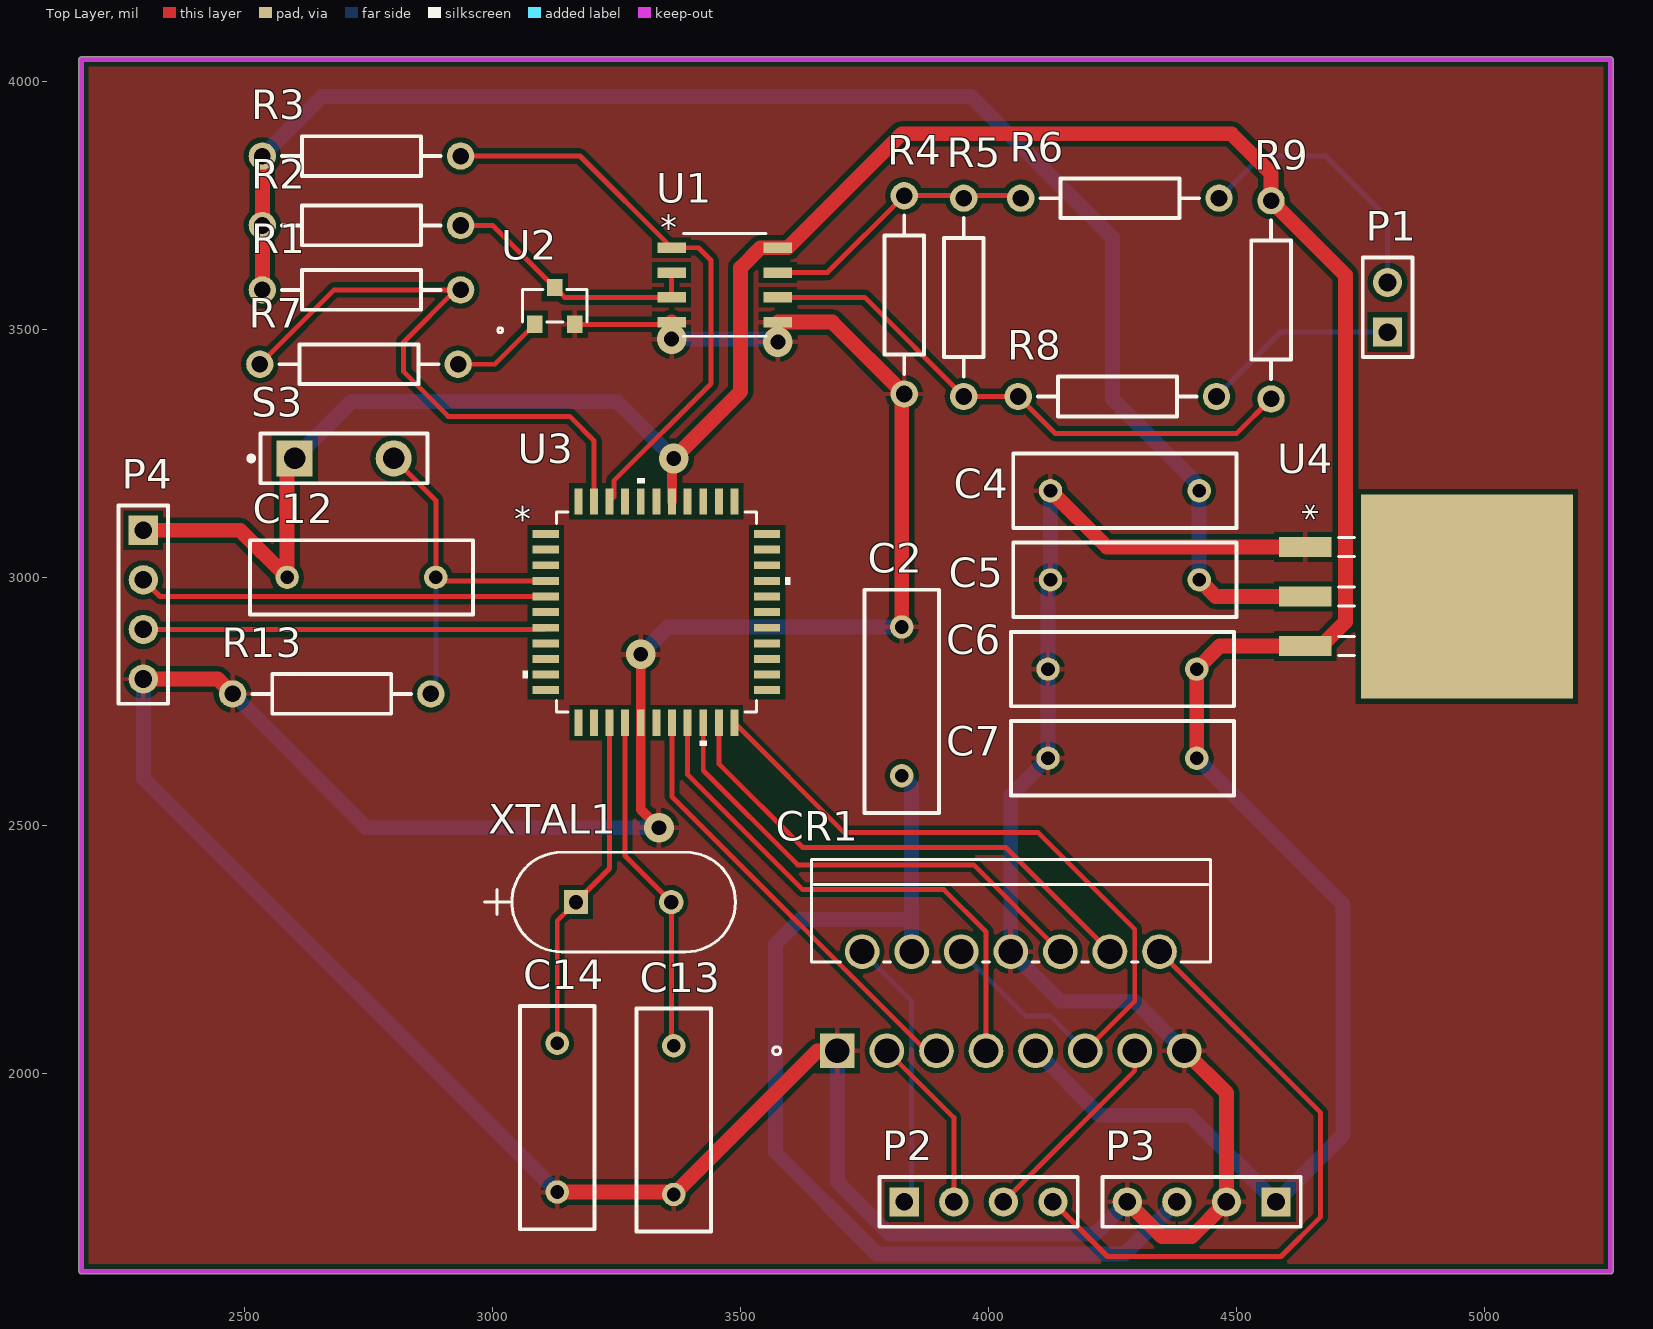
[diagram p0: Top Layer view]
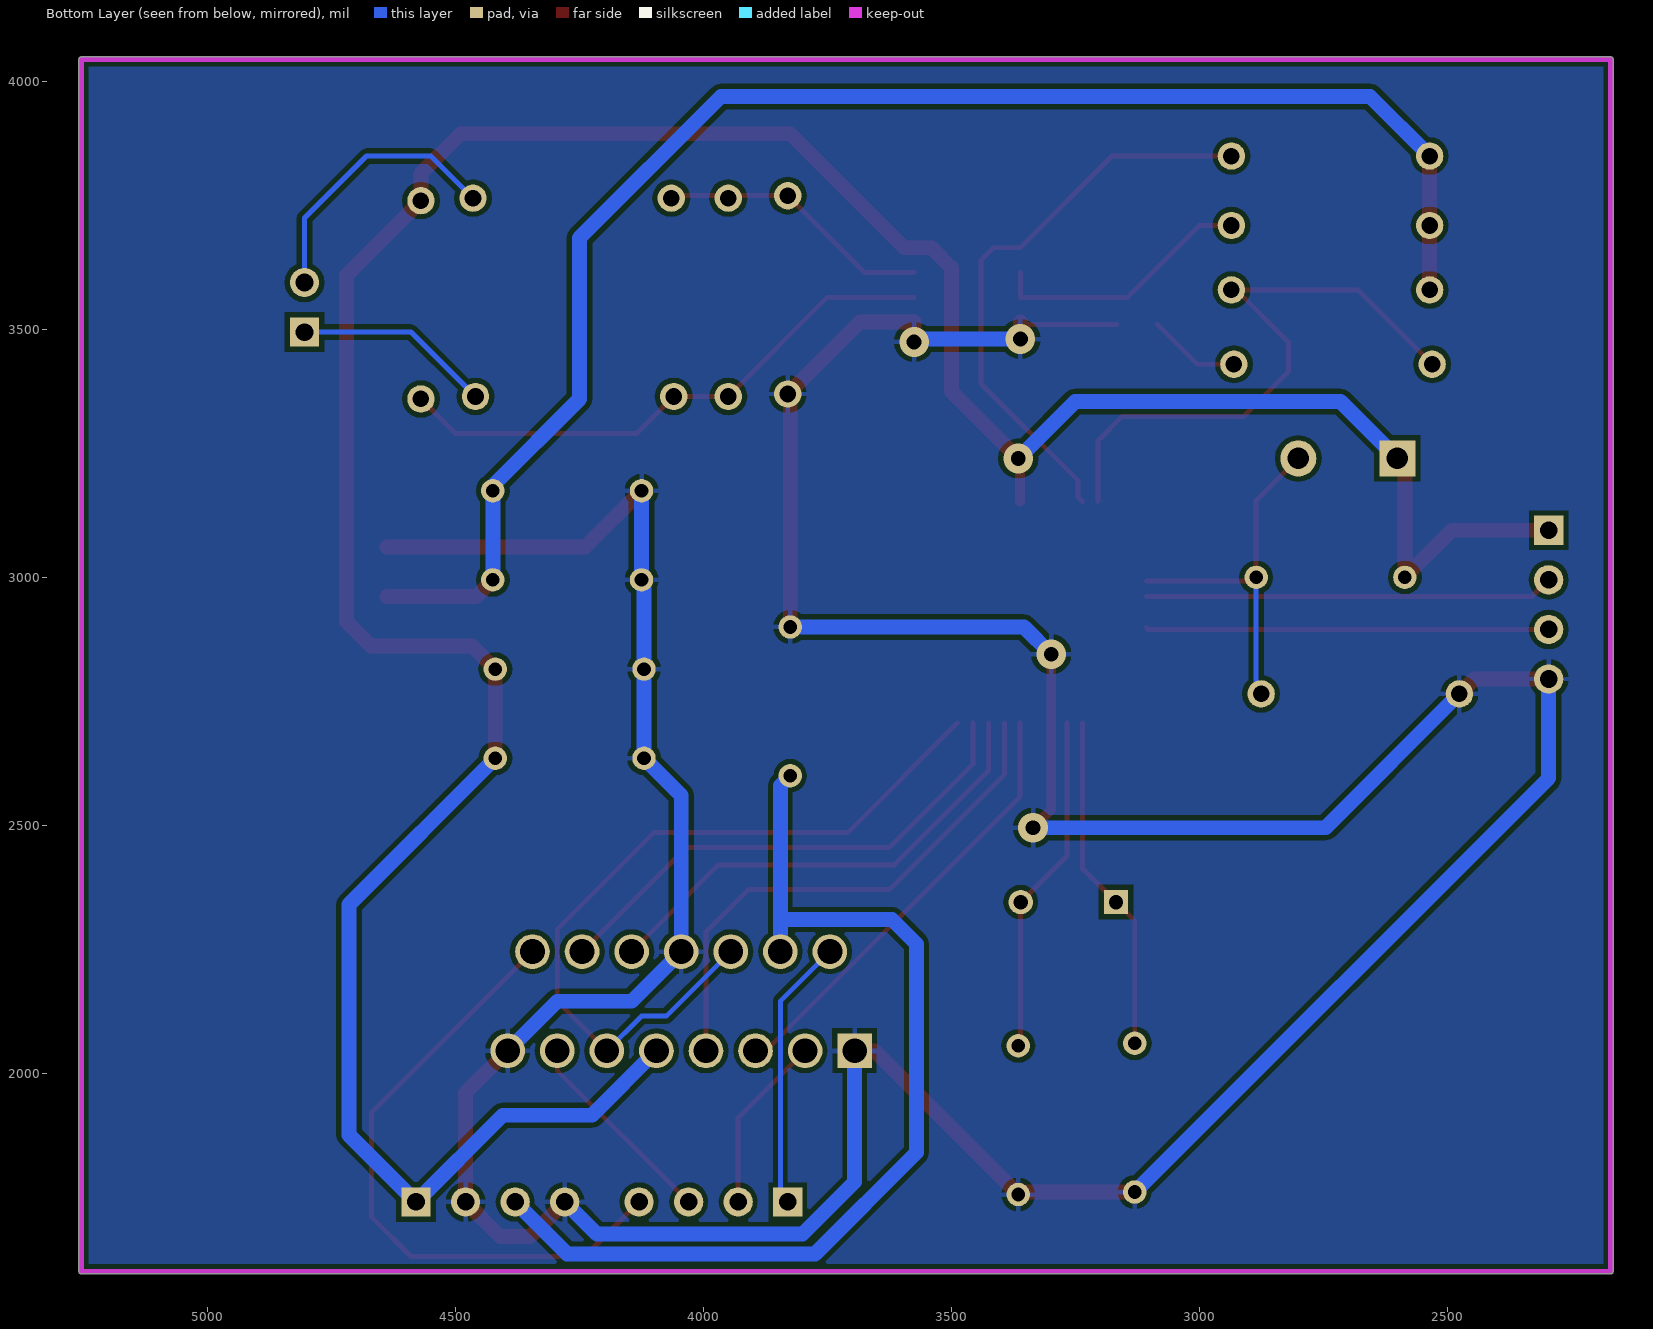
[diagram p1: Bottom Layer view, seen from below]
# Altium PCB MISC76236.PcbDoc
Units mil, origin at the board's own origin, x right, y up, seen from the top; angles counter-clockwise.
Board outline 3095.03 x 2455.03 mil, 2 copper layers (Top Layer, Bottom Layer); 29 components, 26 nets, 128 pads, 5 vias.

## Layer stack, top to bottom (the 12.6 mil dielectric is the usual default, probably not edited)
Top Solder: solder mask 0.4, Solder Resist, Dk 3.5
Top Layer: signal copper 1.4
Dielectric 1: dielectric 12.6, FR-4, Dk 4.8
Bottom Layer: signal copper 1.4
Bottom Solder: solder mask 0.4, Solder Resist, Dk 3.5

## Board outline
2164.99,1600 ccw(c2170,1600) 2170,1594.98 5255,1594.98 ccw(c5255,1600) 5260.02,1600 5260.02,4045 ccw(c5255,4045) 5255,4050.01 2170,4050.01 ccw(c2170,4045) 2164.99,4045

## Design rules (kind name [scope] priority, off if disabled: settings)
Clearance [All] p1: gap=10
MinimumSolderMaskSliver [All] p1: minsoldermaskwidth=0
PolygonConnect [All] p1: connectstyle=Relief reliefconductorwidth=10 reliefentries=4 polygonreliefangle="90 Angle" airgapwidth=10
RoutingVias [All] p1: holewidth=28 width=50 viastyle="Through Hole" minholewidth=28 minwidth=50 maxholewidth=28 maxwidth=50
SilkToSilkClearance [All] p1: silktosilkclearance=0
SilkToSolderMaskClearance [IsPad] p1: minsilkscreentomaskgap=0 clearancetoexposedcopper=TRUE
SolderMaskExpansion [All] p1: expansion=4
Width [All] p1: maxlimit=30 minlimit=10 preferedwidth=10
27 further rules are at their usual default settings.

## Components (designator, comment, footprint, x,y, rotation, side; value= is the part's Value field where it differs from the comment)
C2 "Cap" RAD-0.3 3825,2750 r270 top
C4 "Cap" RAD-0.3 4275,3175 r0 top
C5 "Cap" RAD-0.3 4275,2995 r0 top
C6 "Cap" RAD-0.3 4270,2815 r0 top
C7 "Cap" RAD-0.3 4270,2635 r0 top
C12 "Cap" RAD-0.3 2735,3000 r0 top
C13 "Cap" RAD-0.3 3365,1905 r90 top
C14 "Cap" RAD-0.3 3130,1910 r90 top
CR1 "L298N" Multiwatt15_V_STM 3695,2045 r0 top
P1 "Header 2" HDR1X2 4805,3495 r90 top
P2 "Header 4" HDR1X4 3830,1740 r0 top
P3 "Header 4" HDR1X4 4580,1740 r180 top
P4 "Header 4" HDR1X4 2295,3095 r270 top
R1 "Res2" AXIAL-0.4 2735,3580 r180 top
R2 "Res2" AXIAL-0.4 2735,3710 r180 top
R3 "Res2" AXIAL-0.4 2735,3850 r180 top
R4 "Res2" AXIAL-0.4 3830,3570 r270 top
R5 "Res2" AXIAL-0.4 3950,3565 r90 top
R6 "Res2" AXIAL-0.4 4265,3765 r0 top
R7 "Res2" AXIAL-0.4 2730,3430 r0 top
R8 "Res2" AXIAL-0.4 4260,3365 r0 top
R9 "Res2" AXIAL-0.4 4570,3560 r270 top
R13 "Res2" AXIAL-0.4 2675,2765 r0 top
S3 "SW-PB" SPST-2 2700,3240 r0 top
U1 "MAX485CSA+" 21-0041B_8_MXM 3467.86,3590 r0 top
U2 "MMBT3904-7-F" SOT-23_1_DIO 3125,3547.8 r0 top
U3 "STC12C5A60S2-35I-LQFP44" LQFP44_STC89_STC_SCM 3330,2930 r0 top
U4 "AMS1117-3.3" TS3B_TEX 4965,2961.5 r270 top
XTAL1 "HC49S-11.0592-30-50-70-30-ATF" XTAL_HC49S_MTC 3167.87,2345 r0 top

## Footprints (in the part's own frame and the unit in brackets; to place one, negate y for a bottom-side part, rotate by r counter-clockwise, add the part's x,y. Pads: shape width x height; smd on the part's side, far side on the other; paste and mask are expansions set on the pad)
21-0041B_8_MXM [mil]
  rect 57.28x20.97 smd paste+0 mask+0: 1(-107.14,75) 2(-107.14,25) 3(-107.14,-25) 4(-107.14,-75) 5(107.14,-75) 6(107.14,-25) 7(107.14,25) 8(107.14,75)
  silkscreen extent -84,-104 84,104, body extent -122,-99 122,99, height 69
AXIAL-0.4 [mm] "Axial Device, Thru-Hole; 2 Leads; 0.4 in Pin Spacing"
  round 1.4 hole 0.85: 1(-5.08,0) 2(5.08,0)
  silkscreen extent -4.06,-1.02 4.06,1.02
HDR1X2 [mm] "Connector; Header; 2 Position"
  rect 1.5x1.5 hole 0.9: 1(0,0)
  round 1.5 hole 0.9: 2(2.54,0)
  silkscreen extent -1.27,-1.27 3.81,1.27
HDR1X4 [mm] "Connector; Header; 4 Position"
  rect 1.5x1.5 hole 0.9: 1(0,0)
  round 1.5 hole 0.9: 2(2.54,0) 3(5.08,0) 4(7.62,0)
  silkscreen extent -1.27,-1.27 8.89,1.27
LQFP44_STC89_STC_SCM [mil]
  rect 52.78x15.97 smd paste+0 mask+0: 1(-223.39,157.5) 2(-223.39,126) 3(-223.39,94.5) 4(-223.39,63) 5(-223.39,31.5) 6(-223.39,0) 7(-223.39,-31.5) 8(-223.39,-63) 9(-223.39,-94.5) 10(-223.39,-126) 11(-223.39,-157.5) 23(223.39,-157.5) 24(223.39,-126) 25(223.39,-94.5) 26(223.39,-63) 27(223.39,-31.5) 28(223.39,0) 29(223.39,31.5) 30(223.39,63) 31(223.39,94.5) 32(223.39,126) 33(223.39,157.5)
  rect 15.97x52.78 smd paste+0 mask+0: 12(-157.5,-223.39) 13(-126,-223.39) 14(-94.5,-223.39) 15(-63,-223.39) 16(-31.5,-223.39) 17(0,-223.39) 18(31.5,-223.39) 19(63,-223.39) 20(94.5,-223.39) 21(126,-223.39) 22(157.5,-223.39) 34(157.5,223.39) 35(126,223.39) 36(94.5,223.39) 37(63,223.39) 38(31.5,223.39) 39(0,223.39) 40(-31.5,223.39) 41(-63,223.39) 42(-94.5,223.39) 43(-126,223.39) 44(-157.5,223.39)
  silkscreen extent -270,-270 270,270, body extent -236,-236 236,236, height 63
Multiwatt15_V_STM [mil]
  rect 70x70 / inner round 60 / far side rect 70x70 hole 50 paste-35 mask+0: 1(0,0)
  round 70 / inner round 60 / far side round 70 hole 50 paste-35 mask+0: 2(50,200) 3(100,0) 4(150,200) 5(200,0) 6(250,200) 7(300,0) 8(350,200) 9(400,0) 10(450,200) 11(500,0) 12(550,200) 13(600,0) 14(650,200) 15(700,0)
  silkscreen extent -130,-8 752,386, body extent -48,-15 748,381, height 827
RAD-0.3 [mm] "Radial Cap, Thru-Hole; 2 Leads; 0.3 in Pin Spacing"
  round 1.2 hole 0.7: 1(-3.81,0) 2(3.81,0)
  silkscreen extent -5.71,-1.91 5.71,1.91
SOT-23_1_DIO [mil]
  rect 32x35 smd paste+0 mask+0: 1(-40.35,-37.2) 2(40.35,-37.2) 3(0,37.2)
  silkscreen extent -115,-54 65,33
SPST-2 [mm] "Switch; 2 Leads"
  rect 1.85x1.85 hole 1.1: 1(-2.54,0)
  round 1.85 hole 1.1: 2(2.54,0)
  silkscreen extent -4.89,-1.27 4.28,1.27
TS3B_TEX [mil]
  rect 39.97x105.56 smd paste+0 mask+0: 1(-100,-326) 2(0,-326) 3(100,-326)
  rect 412x428 smd paste+0 mask+0: 4(0,0)
  silkscreen extent -119,-259 119,-227, body extent -205,-278 205,200, height 189
XTAL_HC49S_MTC [mil]
  rect 49x49 / inner round 60 / far side rect 49x49 hole 29 paste-24.5 mask+0: 1(0,0)
  round 49 / inner round 60 / far side round 49 hole 29 paste-24.5 mask+0: 2(192.13,0)
  silkscreen extent -184,-100 322,100, body extent -134,-105 326,105, height 157

## Part data
C2 C4 C5 C6 C7 C12 C13 C14: "Capacitor"
CR1 U1 U2 U3 U4 XTAL1: "No Description Available"
P1: "Header, 2-Pin"
P2 P3 P4: "Header, 4-Pin"
R1 R2 R3 R4 R5 R6 R7 R8 R9 R13: "Resistor"
S3: "Switch"

## Via types
v1: diameter 60, hole 30, Top Layer to Bottom Layer, 5 vias

## Nets (pads, with @x,y where several pads share a name; then routed paths per layer and width w, separated by ;. In a path a pad name is that pad's centre, name@x,y a point inside that pad or via, vN(x,y) a via of type N, cw(c..) or ccw(c..) an arc to the next point about the centre after c; other vN are vias at no path point)
"485 RX": R3.1 U1.1 U3.42 | length 1163.3
  Top Layer w10: R3.1 3175.72,3850 U1.1 3415,3665 3440,3640 3440,3390.76 3244.02,3194.78 3244.02,3161.91 U3.42
"485 TX": R1.1 R7.1 U3.43 | length 1239.8
  Top Layer w10: R7.1 2680,3580 R1.1@2925,3580 ; R1.1 R1.1@2925,3580 ; U3.43 3204,3276 3155,3325 2910,3325 2820,3415 2820,3475 R1.1@2925,3580
+3.3: C4.2 C5.2 R1.2 R2.2 R3.2 U4.2 | length 3143.1
  Top Layer w30: R1.2 R2.2 R3.2 ; C5.2 4458.5,2961.5 U4.2
  Bottom Layer w30: R3.2 2655,3970 3965,3970 4250,3685 4250,3360 4425,3185 C4.2 C5.2
+5: C6.2 C7.2 C12.1 CR1.9 P3.1 P4.1 R9.1 S3.1 U1.8 U3.38 U4.3 | length 6350.7
  Top Layer w20: U3.38 v1@3361.5,3236.5
  Top Layer w30: P4.1 2490,3095 C12.1 2585,3225 S3.1 ; v1@3361.5,3236.5 v1(3365,3240) 3500,3375 3500,3625 3540,3665 U1.8 3595,3665 3825,3895 4490,3895 4570,3815 R9.1 4720,3610 4720,2910 4671.5,2861.5 U4.3 4466.5,2861.5 C6.2 C7.2
  Bottom Layer w30: S3.1 2715,3355 3250,3355 v1(3365,3240) ; CR1.9 4225,1915 4405,1915 P3.1 4715,1875 4715,2340 C7.2
+12: C2.2 CR1.4 P3.3 | length 2017.4
  Bottom Layer w30: C2.2 3845,2580 3845,2310 ; CR1.4 3845,2310 ; P3.3 4275,1635 3775,1635 3570,1840 3570,2260 3620,2310 3845,2310
A: P1.1 R8.2 | length 398.8
  Bottom Layer w10: R8.2 4590,3495 P1.1
A+: CR1.2 P2.1 | length 552.6
  Bottom Layer w10: CR1.2 3845,2145 3845,1755 P2.1
A-: CR1.3 P2.2 | length 360.9
  Top Layer w10: CR1.3 3930,1910 P2.2
B: P1.2 R6.2 | length 557
  Bottom Layer w10: R6.2 4550,3850 4680,3850 4805,3725 P1.2
B+: CR1.13 P2.3 | length 414.8
  Top Layer w10: P2.3 4295,2005 CR1.13
B-: CR1.14 P2.4 | length 1288.3
  Top Layer w10: P2.4 4240,1630 4590,1630 4670,1710 4670,1920 CR1.14
GND: C2.1 C4.1 C5.1 C6.1 C7.1 C13.1 C14.1 CR1.1 CR1.8 CR1.15 P3.2 P3.4 P4.4 R4.2 R13.1 U1.4 U1.5 U2.2 U3.16 U4.1 | length 8897.2
  Top Layer w10: U2.2 3356.31,3510.59 U1.4
  Top Layer w20: v1(3298.5,2845) U3.16 3298.5,2531.5 v1(3335,2495)
  Top Layer w30: P4.4 2445,2795 R13.1 ; C14.1 3360,1760 C13.1 3655,2045 CR1.1 ; v1(3360.72,3480.78) U1.4 ; v1(3575,3475) U1.5 3685,3515 R4.2 3825,3365 C2.1 ; C4.1 4238.5,3061.5 U4.1 ; P3.4 4350,1670 4410,1670 P3.2 4480,1960 CR1.15
  Bottom Layer w30: P4.4 2295,2595 C14.1 ; R13.1 2745,2495 v1(3335,2495) ; v1(3298.5,2845) 3353.5,2900 C2.1 ; v1(3360.72,3480.78) 3569.22,3480.78 v1(3575,3475) ; CR1.1 3695,1780.59 3800.59,1675 4215,1675 P3.4 ; C4.1 C5.1 4120,2990 C6.1 C7.1 4045,2560 CR1.8 4145,2145 4295,2145 CR1.15
NetR2_1: R2.1 U1.2 U1.3 U2.3 | length 535.8
  Top Layer w10: R2.1 3000,3710 U2.3 3145,3565 U1.3 U1.2
NetR4_1: R4.1 R5.2 R6.1 U1.7 | length 556.3
  Top Layer w10: U1.7 3675,3615 R4.1 4060,3770 R6.1
NetR5_1: R5.1 R8.1 R9.2 U1.6 | length 1137.9
  Top Layer w10: U1.6 3750,3565 R5.1 R8.1 4135,3290 4500,3290 R9.2
NetR7_2: R7.2 U2.1 | length 188
  Top Layer w10: R7.2 3004.06,3430 U2.1
P2.0: CR1.5 U3.18 | length 894.7
  Top Layer w10: U3.18 3361.5,2557.79 3874.29,2045 CR1.5
P2.1: CR1.7 U3.19 | length 1077.9
  Top Layer w10: U3.19 3393,2602 3625,2370 3910,2370 3995,2285 CR1.7
P2.2: CR1.10 U3.20 | length 968
  Top Layer w10: U3.20 3424.5,2610.5 3615,2420 3970,2420 CR1.10
P2.3: CR1.12 U3.21 | length 1028.6
  Top Layer w10: U3.21 3456,2624 3625,2455 4035,2455 CR1.12
P2.4: CR1.6 CR1.11 U3.22 | length 1599.3
  Top Layer w10: U3.22 3709.11,2485 4100,2485 4295,2290 4295,2145 CR1.11
  Bottom Layer w10: CR1.6 4075,2115 4125,2115 CR1.11
RESET: C12.2 R13.2 S3.2 U3.4 | length 738.9
  Top Layer w10: S3.2 2885,3155 C12.2 2892,2993 U3.4
  Bottom Layer w10: R13.2 2885,2775 C12.2
RX: P4.2 U3.5 | length 825.7
  Top Layer w10: P4.2 2328.62,2961.38 3106.61,2961.38 U3.5
TX: P4.3 U3.7 | length 813.1
  Top Layer w10: P4.3 3103.11,2895 U3.7
XTAL1: C13.2 U3.15 XTAL1.2 | length 692.2
  Top Layer w10: U3.15 3267,2438 XTAL1.2 3360,2060 C13.2
XTAL2: C14.2 U3.14 XTAL1.1 | length 690.3
  Top Layer w10: C14.2 3130,2307.13 XTAL1.1 3235.5,2412.63 U3.14
pads on no net: U3.1 U3.2 U3.3 U3.6 U3.8 U3.9 U3.10 U3.11 U3.12 U3.13 U3.17 U3.23 U3.24 U3.25 U3.26 U3.27 U3.28 U3.29 U3.30 U3.31 U3.32 U3.33 U3.34 U3.35 U3.36 U3.37 U3.39 U3.40 U3.41 U3.44 U4.4

## Polygon pours and split planes (outlines as drawn)
GND on Bottom Layer "Top Layer-No Net" (solid, remove dead copper, pour order 0): 1715,4360 1720,4355 5915,4355 5915,975 5695,755 5550,900 1675,900
GND on Top Layer "Top Layer-No Net" (solid, remove dead copper, pour order 2): 1765,4360 5720,4360 5770,4410 5435,4075 5435,1280 2055,1280 1955,1180

## Keep-outs
Keep-Out Layer:
  lines w10: 2170,1600 2170,4045 5255,4045 5255,1615 5255,1612.07 5255,1600 4650,1600 2170,1600